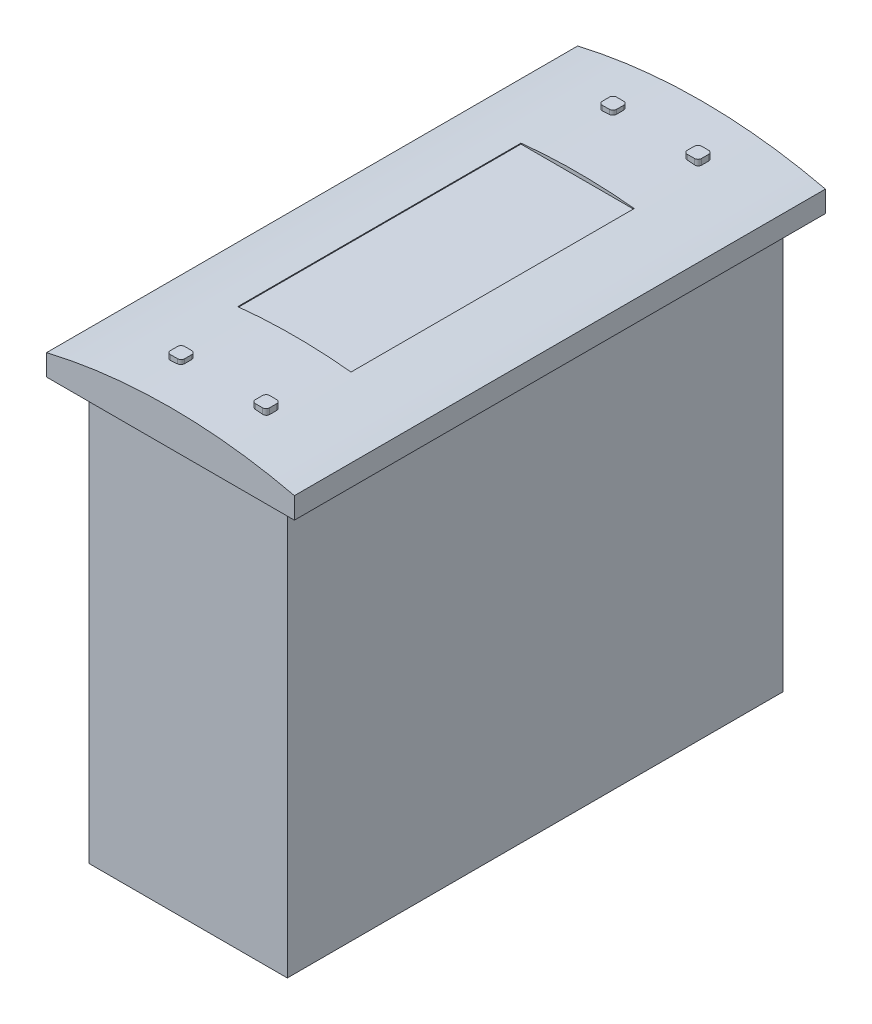
SolidWorks part; units mm, degrees
ref_plane "Front Plane" through (0, 0, 0) normal (0, 0, 1) x (1, 0, 0)
ref_plane "Top Plane" through (0, 0, 0) normal (0, 1, 0) x (1, 0, 0)
ref_plane "Right Plane" through (0, 0, 0) normal (1, 0, 0) x (0, 0, -1)
sketch "Sketch1" plane through (0, 0, 0) normal (0, 0, 1) x (1, 0, 0)
  line L0 (0, 0) -> (35, 0)
  line L1 (35, 0) -> (35, 3)
  line L2 (0, 0) -> (0, 3)
  arc A0 (0, 3) -> (35, 3) centre (17.5, -70.9578) cw
  dimension "D4" = 76
  dimension "D1" = 35
  dimension "D2" = 3
  dimension "D3" = 3
extrude "Boss-Extrude1" add sketch "Sketch1" along normal blind 75
ref_plane "Plane1" through (0, 5.5, 0) normal (0, 1, 0) x (1, 0, 0)
sketch "Sketch2" plane through (0, 5.5, 0) normal (0, 1, 0) x (1, 0, 0)
  line L0 (0, -75) -> (0, 0) construction
  line L1 (9.5, -57.5) -> (25.5, -57.5)
  line L2 (9.5, -57.5) -> (9.5, -17.5)
  line L3 (9.5, -17.5) -> (25.5, -17.5)
  line L4 (25.5, -57.5) -> (25.5, -17.5)
  line L5 (0, -75) -> (35, -75) construction
  dimension "D1" = 40
  dimension "D2" = 16
  dimension "D3" = 9.5
  dimension "D4" = 17.5
extrude "Cut-Extrude1" cut sketch "Sketch2" against normal blind 1
ref_plane "Plane2" through (0, 3, 0) normal (0, -1, 0) x (-1, 0, 0)
sketch "Sketch4" plane through (0, 3, 0) normal (0, -1, 0) x (-1, 0, 0)
  line L0 (-35, -75) -> (0, -75) construction
  line L1 (-11, -69) -> (-13, -69)
  line L2 (-11, -69) -> (-11, -67)
  line L3 (-11, -67) -> (-13, -67)
  line L4 (-13, -69) -> (-13, -67)
  line L5 (-23, -69) -> (-25, -69)
  line L6 (-23, -69) -> (-23, -67)
  line L7 (-23, -67) -> (-25, -67)
  line L8 (-25, -69) -> (-25, -67)
  line L9 (-11, -8) -> (-13, -8)
  line L10 (-11, -8) -> (-11, -6)
  line L11 (-11, -6) -> (-13, -6)
  line L12 (-13, -8) -> (-13, -6)
  line L13 (-23, -8) -> (-25, -8)
  line L14 (-23, -8) -> (-23, -6)
  line L15 (-23, -6) -> (-25, -6)
  line L16 (-25, -8) -> (-25, -6)
  line L17 (-35, -75) -> (-35, 0) construction
  line L18 (0, 0) -> (-35, 0) construction
  dimension "D1" = 2
  dimension "D2" = 2
  dimension "D3" = 2
  dimension "D4" = 2
  dimension "D5" = 6
  dimension "D6" = 6
  dimension "D7" = 10
  dimension "D8" = 10
  dimension "D9" = 2
  dimension "D10" = 2
  dimension "D11" = 2
  dimension "D12" = 2
  dimension "D13" = 10
  dimension "D14" = 10
  dimension "D15" = 6
  dimension "D16" = 6
extrude "Boss-Extrude2" add sketch "Sketch4" against normal blind 2.5 separate body
fillet "Fillet1" radius 0.5 4 edges at (13, 4.25, 69) (13, 4.25, 67) (11, 4.25, 67) (11, 4.25, 69)
fillet "Fillet2" radius 0.5 4 edges at (25, 4.25, 69) (25, 4.25, 67) (23, 4.25, 67) (23, 4.25, 69)
fillet "Fillet3" radius 0.5 4 edges at (11, 4.25, 8) (13, 4.25, 8) (13, 4.25, 6) (11, 4.25, 6)
fillet "Fillet4" radius 0.5 4 edges at (25, 4.25, 8) (23, 4.25, 8) (25, 4.25, 6) (23, 4.25, 6)
sketch "Sketch5" plane through (0, 0, 0) normal (0, -1, 0) x (1, 0, 0)
  line L0 (0, 0) -> (35, 0) construction
  line L1 (3.5, 2.5) -> (31.5, 2.5)
  line L2 (3.5, 2.5) -> (3.5, 72.5)
  line L3 (3.5, 72.5) -> (31.5, 72.5)
  line L4 (31.5, 2.5) -> (31.5, 72.5)
  line L5 (35, 75) -> (35, 0) construction
  dimension "D1" = 28
  dimension "D2" = 70
  dimension "D3" = 2.5
  dimension "D4" = 3.5
extrude "Boss-Extrude3" add sketch "Sketch5" along normal blind 59
